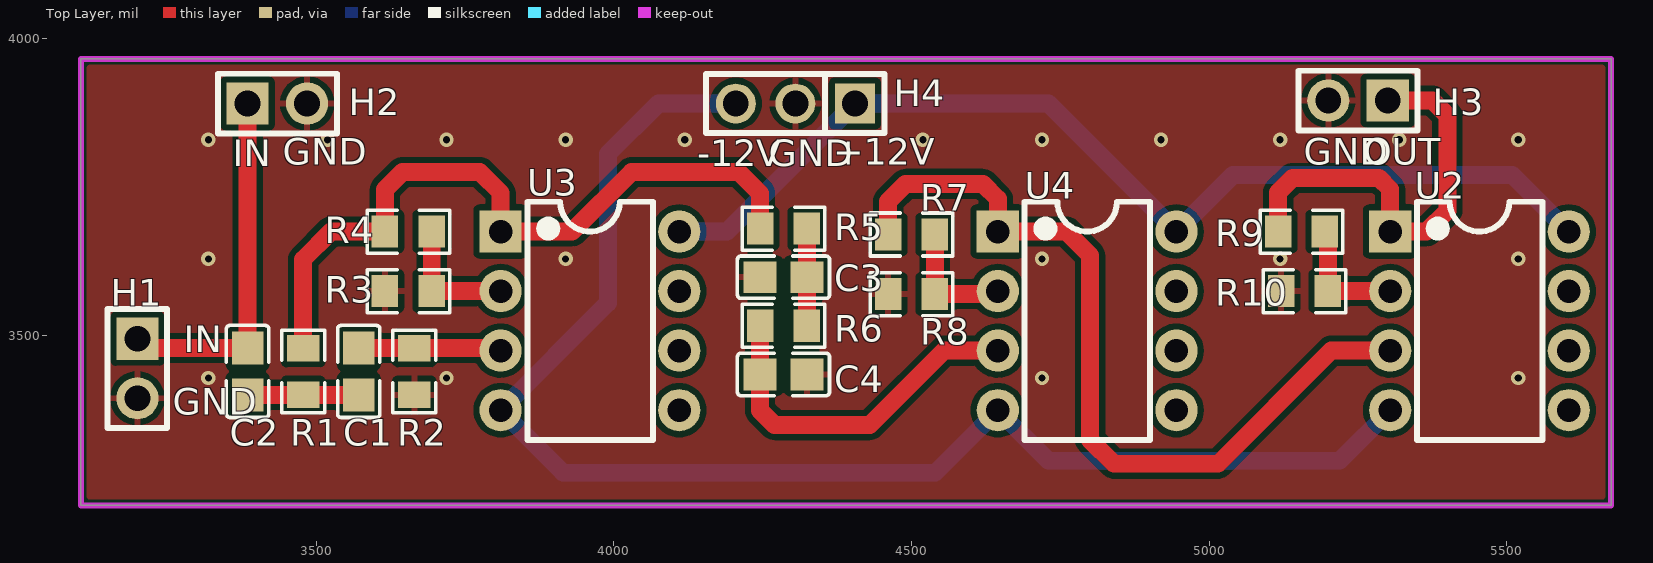
[diagram p0: Top Layer view]
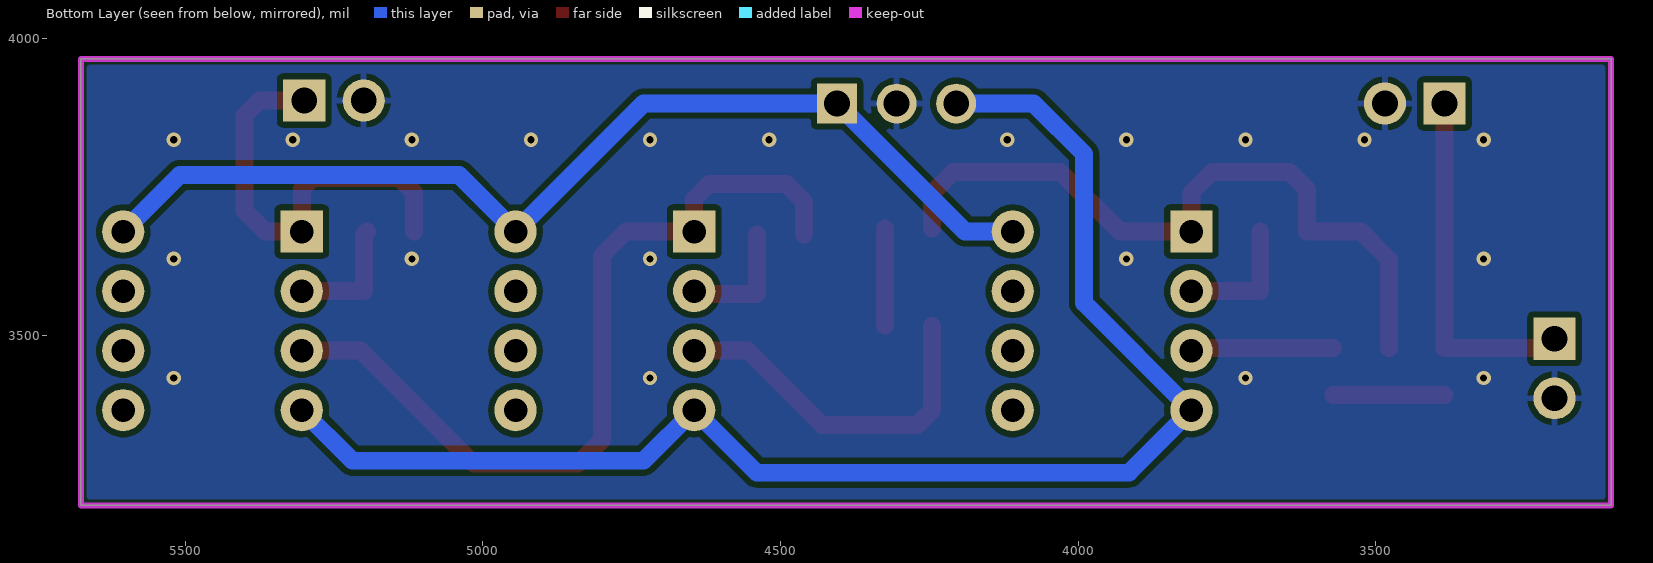
[diagram p1: Bottom Layer view, seen from below]
# Altium PCB MISC51939.pcbdoc
Units mil, origin at the board's own origin, x right, y up, seen from the top; angles counter-clockwise.
Board outline 2570 x 750 mil, 2 copper layers (Top Layer, Bottom Layer), stack 62.206 mil thick; 21 components, 14 nets, 61 pads, 20 vias.

## Layer stack, top to bottom
Top Solder Mask Layer: solder mask 0.394, Dk 3.3
Top Layer: signal copper 1.379
Dielectric1: surface 59.449, FR4, Dk 4.5
Bottom Layer: signal copper 1.378
Bottom Solder Mask Layer: solder mask 0.394, Dk 3.3

## Board outline
3105,3965 3105,3215 5675,3215 5675,3965

## Design rules (kind name [scope] priority, off if disabled: settings)
BoardOutlineClearance copperThickness2oz_1 [All] p2 off: genericclearance=7.99 ignorepadtopadclearanceinfootprint=FALSE except(0: Arc-SplitContinuation Track-SplitContinuation SMDPad-SplitContinuation THPad-SplitContinuation Via-SplitContinuation Fill-SplitContinuation Region-SplitContinuation Poly-SplitContinuation Text-SplitContinuation Hole-SplitContinuation; 5.98: Arc-CutoutEdge SMDPad-CutoutEdge THPad-CutoutEdge Via-CutoutEdge Fill-CutoutEdge Region-CutoutEdge Text-CutoutEdge; 6.93: Hole-OutlineEdge Hole-CutoutEdge; 10: Poly-OutlineEdge Poly-CutoutEdge; 11.81: Arc-OutlineEdge Track-OutlineEdge SMDPad-OutlineEdge THPad-OutlineEdge Via-OutlineEdge Fill-OutlineEdge Region-OutlineEdge Text-OutlineEdge Track-CutoutEdge)
BoardOutlineClearance copperThickness1oz_1 [All] p4: genericclearance=4.02 ignorepadtopadclearanceinfootprint=FALSE except(0: Arc-SplitContinuation Track-SplitContinuation SMDPad-SplitContinuation THPad-SplitContinuation Via-SplitContinuation Fill-SplitContinuation Region-SplitContinuation Poly-SplitContinuation Text-SplitContinuation Hole-SplitContinuation; 6: SMDPad-CutoutEdge THPad-CutoutEdge Via-CutoutEdge Fill-CutoutEdge Region-CutoutEdge Text-CutoutEdge; 6.93: Hole-OutlineEdge Hole-CutoutEdge; 10: Poly-OutlineEdge Poly-CutoutEdge; 11.8: Arc-OutlineEdge Track-OutlineEdge SMDPad-OutlineEdge THPad-OutlineEdge Via-OutlineEdge Fill-OutlineEdge Region-OutlineEdge Text-OutlineEdge; 11.81: Arc-CutoutEdge Track-CutoutEdge)
Clearance copperThickness2oz [All] p1 off: gap=7.99 ignorepadtopadclearanceinfootprint=FALSE except(5.98: SMDPad-Track SMDPad-SMDPad THPad-Track SMDPad-THPad THPad-THPad Track-Via SMDPad-Via THPad-Via Via-Via Fill-Track Region-Track Fill-SMDPad Region-SMDPad Fill-THPad Region-THPad Fill-Via Region-Via Fill-Fill Fill-Region Region-Region Arc-Track Arc-SMDPad Arc-THPad Arc-Via Fill-Arc Region-Arc Arc-Arc Text-Track SMDPad-Text Text-THPad Text-Via Fill-Text Region-Text Arc-Text Text-Text; 6.93: Hole-Track Hole-SMDPad Hole-THPad Hole-Via Fill-Hole Region-Hole Hole-Arc Hole-Text; 10: Poly-Track Poly-SMDPad Poly-THPad Poly-Via Poly-Fill Poly-Region Poly-Poly Poly-Arc Poly-Text Poly-Hole)
Clearance copperThickness1oz [All] p3: gap=4.02 ignorepadtopadclearanceinfootprint=FALSE except(5.98: SMDPad-Track SMDPad-SMDPad THPad-Track SMDPad-THPad THPad-THPad Track-Via SMDPad-Via THPad-Via Via-Via Fill-Track Region-Track Fill-SMDPad Region-SMDPad Fill-THPad Region-THPad Fill-Via Region-Via Fill-Fill Fill-Region Region-Region; 6: Arc-Track Arc-SMDPad Arc-THPad Arc-Via Fill-Arc Region-Arc Arc-Arc Text-Track SMDPad-Text Text-THPad Text-Via Fill-Text Region-Text Arc-Text Text-Text; 6.93: Hole-Track Hole-SMDPad Hole-THPad Hole-Via Fill-Hole Region-Hole Hole-Arc Hole-Text; 10: Poly-Track Poly-SMDPad Poly-THPad Poly-Via Poly-Fill Poly-Region Poly-Poly Poly-Arc Poly-Text Poly-Hole)
DiffPairsRouting differentialPair [All] p1: maxlimit=6 minlimit=6 mostfreqgap=6 toplayer_minwidth=5 toplayer_prefwidth=10 toplayer_maxwidth=100 toplayer_mingap=6 toplayer_prefgap=6 toplayer_maxgap=6 bottomlayer_minwidth=5 bottomlayer_prefwidth=10 bottomlayer_maxwidth=100 bottomlayer_mingap=6 bottomlayer_prefgap=6 bottomlayer_maxgap=6 maxuncoupledlength=10
HoleToHoleClearance otherClearance [All] p1: gap=11.81 allowstackedmicrovias=TRUE
Length netLength [All] p1: minlimit=0 maxlimit=0
MatchedLengths netLengthTolerance [All] p1: tolerance=1000
PasteMaskExpansion pasteMaskExpansion [All] p1: expansion=0
PlaneConnect innerPlane [All] p1: planeconnectstyle=Relief reliefexpansion=20 reliefentries=4 reliefconductorwidth=10 reliefairgap=10
PolygonConnect copperRegion [(InNet('GND'))] p1: connectstyle=Relief reliefconductorwidth=10 reliefentries=4 polygonreliefangle="90 Angle" airgapwidth=10 via.connectstyle=Relief via.reliefconductorwidth=10 via.reliefentries=4 via.polygonreliefangle="90 Angle" via.airgapwidth=10
RoutingVias viaSize [All] p1: holewidth=12.01 width=24.02 viastyle="Through Hole" minholewidth=11.81 minwidth=19.68 maxholewidth=248.03 maxwidth=393.7
SolderMaskExpansion solderMaskExpansion [IsVia] p1: expansion=-1000 istentingtop=TRUE
SolderMaskExpansion solderMaskExpansion [All] p2: expansion=2 istentingtop=FALSE
Width copperThickness2oz_2 [All] p1 off: maxlimit=100 minlimit=8 preferedwidth=10
Width copperThickness1oz_2 [All] p2: maxlimit=100 minlimit=5 preferedwidth=10

## Components (designator, comment, footprint, x,y, rotation, side; value= is the part's Value field where it differs from the comment)
C1 "10uF" C0805 3571.67,3440 r90 top
C2 "10uF" C0805 3385,3440 r270 top
C3 "1nF" C0805 4285,3598.33 r0 top
C4 "1nF" C0805 4285,3435 r180 top
H1 "" HDR-TH_2P-P2.54-V-M-1 3200,3445 r270 top
H2 "" HDR-TH_2P-P2.54-V-M-1 3435,3890 r0 top
H3 "" HDR-TH_2P-P2.54-V-M-1 5250,3895 r180 top
H4 "" HDR-TH_3P-P2.54-V-M 4305,3890 r180 top
R1 "2.6K" R0805 3478.33,3440 r270 top
R2 "2.6K" R0805 3665,3440 r90 top
R3 "10K" R0805 3655,3575 r0 top
R4 "10K" R0805 3655,3675 r180 top
R5 "5.1K" R0805 4285,3680 r0 top
R6 "5.1K" R0805 4285,3516.67 r180 top
R7 "10K" R0805 4500,3670 r180 top
R8 "10K" R0805 4500,3570 r0 top
R9 "24K" R0805 5155,3675 r180 top
R10 "1K" R0805 5160,3575 r0 top
U2 "LM358AD" PDIP-8_L9.5-W6.4-P2.54-LS7.6-BL 5453.92,3525 r270 top
U3 "LM358AD" PDIP-8_L9.5-W6.4-P2.54-LS7.6-BL 3960,3525 r270 top
U4 "LM358AD" PDIP-8_L9.5-W6.4-P2.54-LS7.6-BL 4795,3525 r270 top

## Footprints (in the part's own frame and the unit in brackets; to place one, negate y for a bottom-side part, rotate by r counter-clockwise, add the part's x,y. Pads: shape width x height; smd on the part's side, far side on the other; paste and mask are expansions set on the pad)
C0805 [mm]
  rect 1.41x1.35 smd paste-100 mask+0.051: 1(-1,0) 2(1,0)
  silkscreen extent -1.96,-0.9 1.96,0.9
HDR-TH_2P-P2.54-V-M-1 [mm]
  rect 1.8x1.8 hole 1.1: 1(-1.27,0)
  round 1.8 hole 1.1: 2(1.27,0)
  silkscreen extent -2.54,-1.27 2.54,1.27
HDR-TH_3P-P2.54-V-M [mm]
  rect 1.7x1.7 hole 1.1: 1(-2.54,0)
  round 1.7 hole 1.1: 2(0,0) 3(2.54,0)
  silkscreen extent -3.81,-1.25 3.81,1.25
PDIP-8_L9.5-W6.4-P2.54-LS7.6-BL [mm]
  rect 1.8x1.8 hole 1: 1(-3.81,-3.81)
  round 1.8 hole 1: 2(-1.27,-3.81) 3(1.27,-3.81) 4(3.81,-3.81) 5(3.81,3.81) 6(1.27,3.81) 7(-1.27,3.81) 8(-3.81,3.81)
  silkscreen extent -5.08,-2.67 5.08,2.68
R0805 [mm]
  rect 1.133x1.377 smd paste-100 mask+0.051: 1(-1,0) 2(1,0)
  silkscreen extent -1.76,-0.92 1.76,0.92

## Via types
v1: diameter 24.02, hole 12, Top Layer to Bottom Layer, 20 vias

## Nets (pads, with @x,y where several pads share a name; then routed paths per layer and width w, separated by ;. In a path a pad name is that pad's centre, name@x,y a point inside that pad or via, vN(x,y) a via of type N, cw(c..) or ccw(c..) an arc to the next point about the centre after c; other vN are vias at no path point)
12V: H4.1 U2.8 U3.8 U4.8 | length 1750.7
  Bottom Layer w30: U3.8 4190,3675 H4.1 4730,3890 U4.8 5040,3770 5508.92,3770 U2.8
$1N4: C1.2 R2.2 U3.3 | length 240.1
  Top Layer w30: C1.2 R2.2 3805.63,3479.37 U3.3
$1N5: C1.1 C2.2 R1.2 | length 186.7
  Top Layer w30: C2.2 R1.2 C1.1
$1N7: R1.1 R4.2 R5.1 U3.1 | length 1213.4
  Top Layer w30: R1.1 3478.33,3628.33 3525,3675 R4.2 3615.63,3745.63 3645,3775 3775,3775 3810,3740 U3.1 3930,3675 4030,3775 4210,3775 4245.63,3739.37 R5.1
$1N8: R3.2 R4.1 U3.2 | length 215.6
  Top Layer w30: R4.1 R3.2 U3.2
$1N10: C2.1 H1.1 H2.1 | length 602.1
  Top Layer w30: H1.1 3215.63,3479.37 C2.1 H2.1
$1N15: C3.2 R5.2 R6.1 | length 163.3
  Top Layer w30: R6.1 C3.2 R5.2
$1N18: C4.2 R6.2 U4.3 | length 603.5
  Top Layer w30: R6.2 C4.2 4245.63,3374.37 4270,3350 4430,3350 4555,3475 U4.3
$1N19: R7.1 R8.2 U4.2 | length 207.7
  Top Layer w30: R7.1 R8.2 4640,3570 U4.2
$1N21: R7.2 U2.3 U4.1 | length 1398.3
  Top Layer w30: R7.2 4460.63,3725.63 4490,3755 4620,3755 4645,3730 U4.1 4760,3675 4800,3635 4800,3325 4840,3285 5015,3285 5205,3475 U2.3
$1N22: R9.1 R10.2 U2.2 | length 206.6
  Top Layer w30: R9.1 5199.37,3670 R10.2 U2.2
$1N24: H3.1 R9.2 U2.1 | length 723.9
  Top Layer w30: R9.2 5115.63,3740.63 5140,3765 5285,3765 5303.92,3746.08 U2.1 5365,3675 5400,3710 5400,3870 5375,3895 H3.1
-12V: H4.3 U2.4 U3.4 U4.4 | length 2406.1
  Bottom Layer w30: H4.3 4075,3890 3990,3805 3990,3555 U3.4 3915,3270 4540,3270 U4.4 4730,3290 5218.92,3290 U2.4
GND: C3.1 C4.1 H1.2 H2.2 H3.2 H4.2 R2.1 R3.1 R8.1 R10.1
  other v1: 3319.1,3429.1 3719.1,3429.1 4719.1,3429.1 5519.1,3429.1 3319.1,3629.1 3919.1,3629.1 4719.1,3629.1 5119.1,3629.1 5519.1,3629.1 3319.1,3829.1 3519.1,3829.1 3719.1,3829.1 3919.1,3829.1 4119.1,3829.1 4519.1,3829.1 4719.1,3829.1 4919.1,3829.1 5119.1,3829.1 5319.1,3829.1 5519.1,3829.1
pads on no net: U2.5 U2.6 U2.7 U3.5 U3.6 U3.7 U4.5 U4.6 U4.7

## Polygon pours and split planes (outlines as drawn)
GND on Top Layer (solid, remove dead copper, pour order 0): 3000,4180 3000,3000 5875,3000 5875,4180
GND on Bottom Layer (solid, remove dead copper, pour order 2): 3020,4135 3020,3075 5785,3075 5785,4135

## Keep-outs
Board Outline Layer:
  the board outline again, w10

## Silkscreen, mask and mechanical layers (free items; w line width, h text height)
Top Silkscreen Layer:
  text "GND" at 3443.95,3787.5 h45
  text "+12V" at 4368.95,3787.5 h45
  text "GND" at 5158.95,3787.5 h45
  text "OUT" at 5258.95,3787.5 h45
  text "IN" at 3360,3785 h45
  text "-12V" at 4140,3785 h45
  text "GND" at 4260,3785 h45
  text "IN" at 3277.55,3472.5 h45
  text "GND" at 3258.95,3367.5 h45